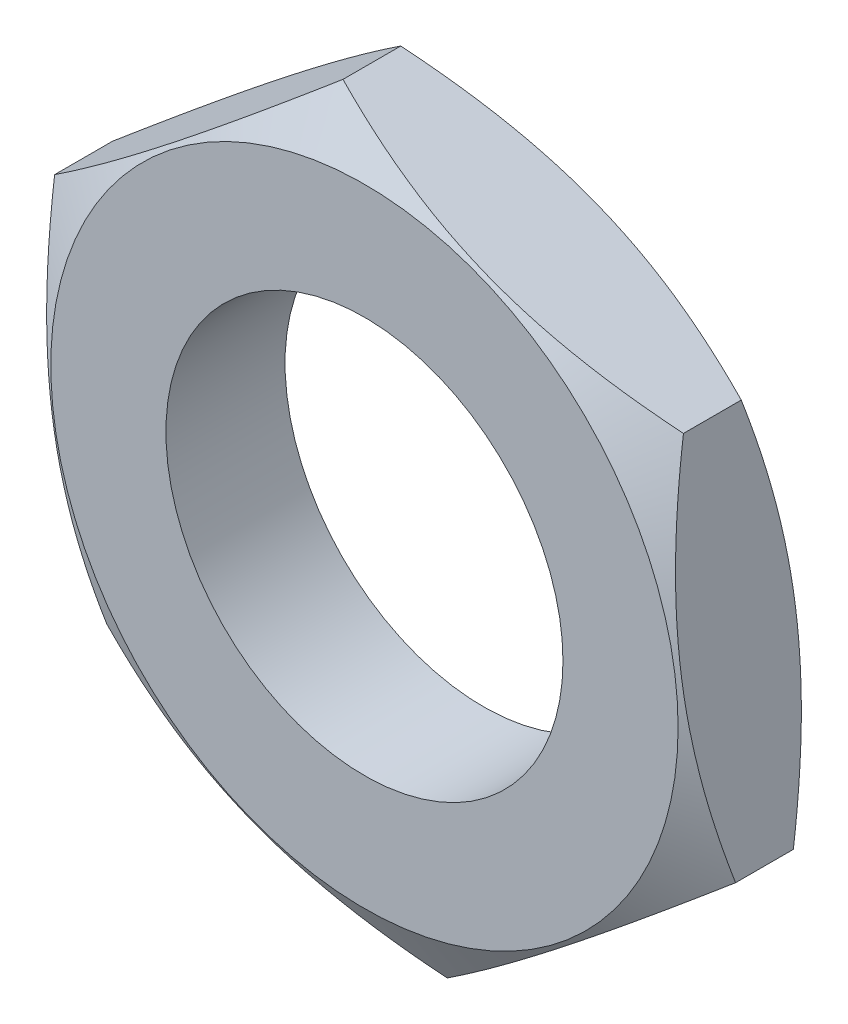
from build123d import *

# Parameters (mm, degrees)
SKETCH1_R           = 10
BOSS_EXTRUDE1_DEPTH = 6
SKETCH3_OUTSIDE_W   = 81.044
SKETCH3_OUTSIDE_H   = 83.318
SKETCH3_OUTSIDE_R   = 15.8
CUT_EXTRUDE2_DEPTH  = 10
CUT_EXTRUDE2_DRAFT  = -60
SKETCH4_OUTSIDE_W   = 63.722
SKETCH4_OUTSIDE_H   = 65.996
SKETCH4_OUTSIDE_R   = 15.8
CUT_EXTRUDE3_DEPTH  = 5
CUT_EXTRUDE3_DRAFT  = -60


with BuildPart() as part:
    # Sketch1 → Boss-Extrude1 (new body)
    with BuildSketch(Plane.XY):
        Polygon((-14.524594865, -11.417945408), (2.62593335, -18.287640837), (17.150528215, -6.869695429), (14.524594865, 11.417945408), (-2.62593335, 18.287640837), (-17.150528215, 6.869695429), align=None)
        Circle(SKETCH1_R, mode=Mode.SUBTRACT)
    extrude(amount=BOSS_EXTRUDE1_DEPTH)


with BuildPart() as cut_extrude2_tool:
    # Sketch3 outside → Cut-Extrude2 (with draft: the straight prism first)
    with BuildSketch(Plane.XY.offset(6)):
        Rectangle(SKETCH3_OUTSIDE_W, SKETCH3_OUTSIDE_H)
        Circle(SKETCH3_OUTSIDE_R, mode=Mode.SUBTRACT)
    extrude(amount=-CUT_EXTRUDE2_DEPTH)
    # Cut-Extrude2: the draft: its side faces are tilted about the plane it starts from
    cut_extrude2_sides = [cut_extrude2_tool.faces().sort_by_distance(p)[0] for p in [
        (0, -41.659, 1),
        (40.522, 0, 1),
        (0, 41.659, 1),
        (-40.522, 0, 1),
        (-15.8, 0, 1),
    ]]
    draft(cut_extrude2_sides, Plane.XY.offset(6), CUT_EXTRUDE2_DRAFT)


with BuildPart() as part_1:
    add(part.part)

    # Cut-Extrude2: cut by cut_extrude2_tool
    add(cut_extrude2_tool.part, mode=Mode.SUBTRACT)


with BuildPart() as cut_extrude3_tool:
    # Sketch4 outside → Cut-Extrude3 (with draft: the straight prism first)
    with BuildSketch(Plane(origin=(0, 0, 0), x_dir=(-1, 0, 0), z_dir=(0, 0, -1))):
        Rectangle(SKETCH4_OUTSIDE_W, SKETCH4_OUTSIDE_H)
        Circle(SKETCH4_OUTSIDE_R, mode=Mode.SUBTRACT)
    extrude(amount=-CUT_EXTRUDE3_DEPTH)
    # Cut-Extrude3: the draft: its side faces are tilted about the plane it starts from
    cut_extrude3_sides = [cut_extrude3_tool.faces().sort_by_distance(p)[0] for p in [
        (0, -32.998, 2.5),
        (-31.861, 0, 2.5),
        (0, 32.998, 2.5),
        (31.861, 0, 2.5),
        (15.8, 0, 2.5),
    ]]
    draft(cut_extrude3_sides, Plane(origin=(0, 0, 0), x_dir=(-1, 0, 0), z_dir=(0, 0, -1)), CUT_EXTRUDE3_DRAFT)


with BuildPart() as part_2:
    add(part_1.part)

    # Cut-Extrude3: cut by cut_extrude3_tool
    add(cut_extrude3_tool.part, mode=Mode.SUBTRACT)


solid = part_2.part
